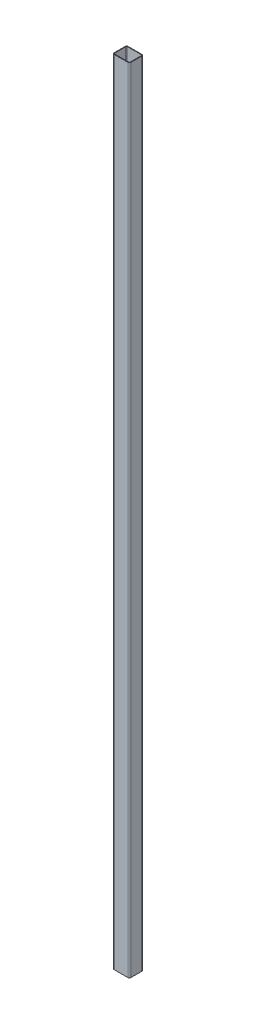
from build123d import *

# Parameters (mm, degrees)
EXTRUDE_THIN1_DEPTH = 2851


with BuildPart() as part:
    # Sketch1 → Extrude-Thin1 (new, symmetric)
    with BuildSketch(Plane(origin=(0, 0, 0), x_dir=(1, 0, 0), z_dir=(0, 1, 0))):
        with BuildLine():
            Line((-50, 50), (50, 50))
            ThreePointArc((50, 50), (57.071067812, 47.071067812), (60, 40))
            Line((60, 40), (60, -40))
            ThreePointArc((60, -40), (57.071067812, -47.071067812), (50, -50))
            Line((50, -50), (-50, -50))
            ThreePointArc((-50, -50), (-57.071067812, -47.071067812), (-60, -40))
            Line((-60, -40), (-60, 40))
            ThreePointArc((-60, 40), (-57.071067812, 47.071067812), (-50, 50))
        make_face()
        with BuildLine():
            Line((-50, 46), (50, 46))
            ThreePointArc((50, 46), (54.242640687, 44.242640687), (56, 40))
            Line((56, 40), (56, -40))
            ThreePointArc((56, -40), (54.242640687, -44.242640687), (50, -46))
            Line((50, -46), (-50, -46))
            ThreePointArc((-50, -46), (-54.242640687, -44.242640687), (-56, -40))
            Line((-56, -40), (-56, 40))
            ThreePointArc((-56, 40), (-54.242640687, 44.242640687), (-50, 46))
        make_face(mode=Mode.SUBTRACT)
    extrude(amount=EXTRUDE_THIN1_DEPTH, both=True)


solid = part.part
